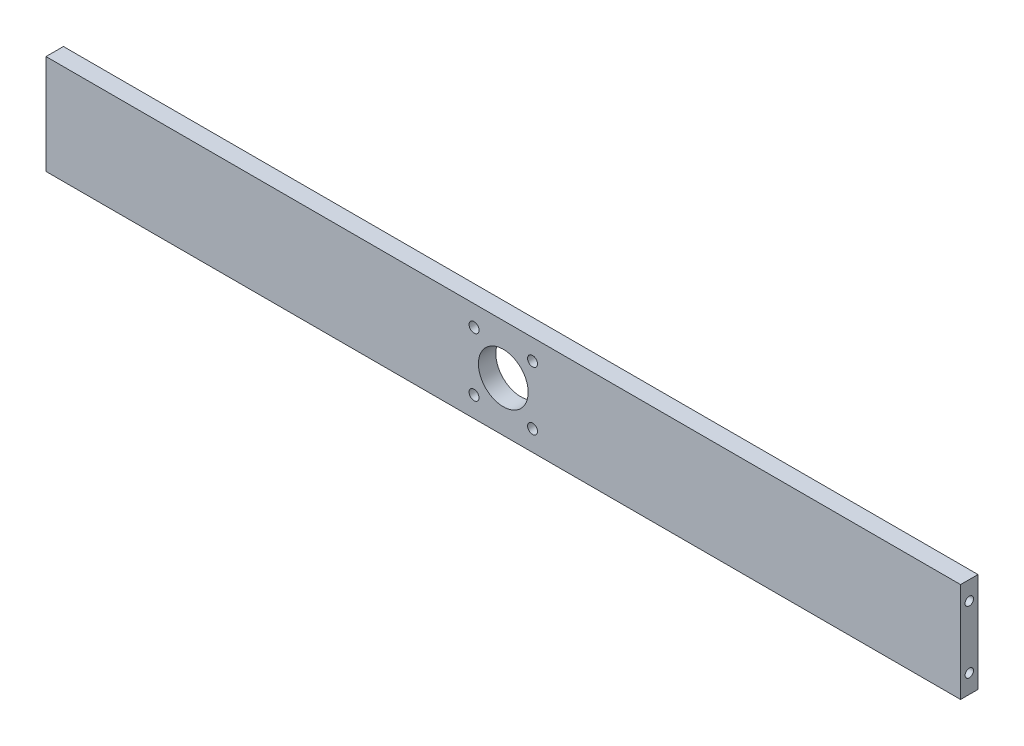
from build123d import *

# Parameters (mm, degrees)
SKETCH1_W             = 735
SKETCH1_H             = 80
BOSS_EXTRUDE1_DEPTH   = 14
SKETCH2_R             = 4
SKETCH2_R_2           = 20
CUT_EXTRUDE1_DEPTH    = 14
M8_TAPPED_HOLE1_D     = 6.8
M8_TAPPED_HOLE1_DEPTH = 19.75
M8_TAPPED_HOLE1_TIP   = 2.042926105
M8_TAPPED_HOLE2_D     = 6.8
M8_TAPPED_HOLE2_DEPTH = 19.75
M8_TAPPED_HOLE2_TIP   = 2.042926105


with BuildPart() as part:
    # Sketch1 → Boss-Extrude1 (new body)
    with BuildSketch(Plane.XY):
        with Locations((367.5, 40)):
            Rectangle(SKETCH1_W, SKETCH1_H)
    extrude(amount=BOSS_EXTRUDE1_DEPTH)

    # Sketch2 → Cut-Extrude1 (cut)
    with BuildSketch(Plane.XY.offset(14)):
        with Locations((344, 63.5)):
            Circle(SKETCH2_R)
        with Locations((344, 16.5)):
            Circle(SKETCH2_R)
        with Locations((391, 16.5)):
            Circle(SKETCH2_R)
        with Locations((391, 63.5)):
            Circle(SKETCH2_R)
        with Locations((367.5, 40)):
            Circle(SKETCH2_R_2)
    extrude(amount=-CUT_EXTRUDE1_DEPTH, mode=Mode.SUBTRACT)

    # M8 Tapped Hole1
    with Locations(Plane(origin=(0, 65, 7), x_dir=(0, 0, -1), z_dir=(-1, 0, 0))):
        with Locations((0, 0), (0, 50)):
            Hole(M8_TAPPED_HOLE1_D / 2, depth=M8_TAPPED_HOLE1_DEPTH)
            with Locations((0, 0, -(M8_TAPPED_HOLE1_DEPTH + M8_TAPPED_HOLE1_TIP / 2))):  # 118° drill point
                Cone(0, M8_TAPPED_HOLE1_D / 2, M8_TAPPED_HOLE1_TIP, mode=Mode.SUBTRACT)

    # M8 Tapped Hole2
    with Locations(Plane(origin=(735, 15, 7), x_dir=(0, 0, 1), z_dir=(1, 0, 0))):
        with Locations((0, 0), (0, -50)):
            Hole(M8_TAPPED_HOLE2_D / 2, depth=M8_TAPPED_HOLE2_DEPTH)
            with Locations((0, 0, -(M8_TAPPED_HOLE2_DEPTH + M8_TAPPED_HOLE2_TIP / 2))):  # 118° drill point
                Cone(0, M8_TAPPED_HOLE2_D / 2, M8_TAPPED_HOLE2_TIP, mode=Mode.SUBTRACT)


solid = part.part
